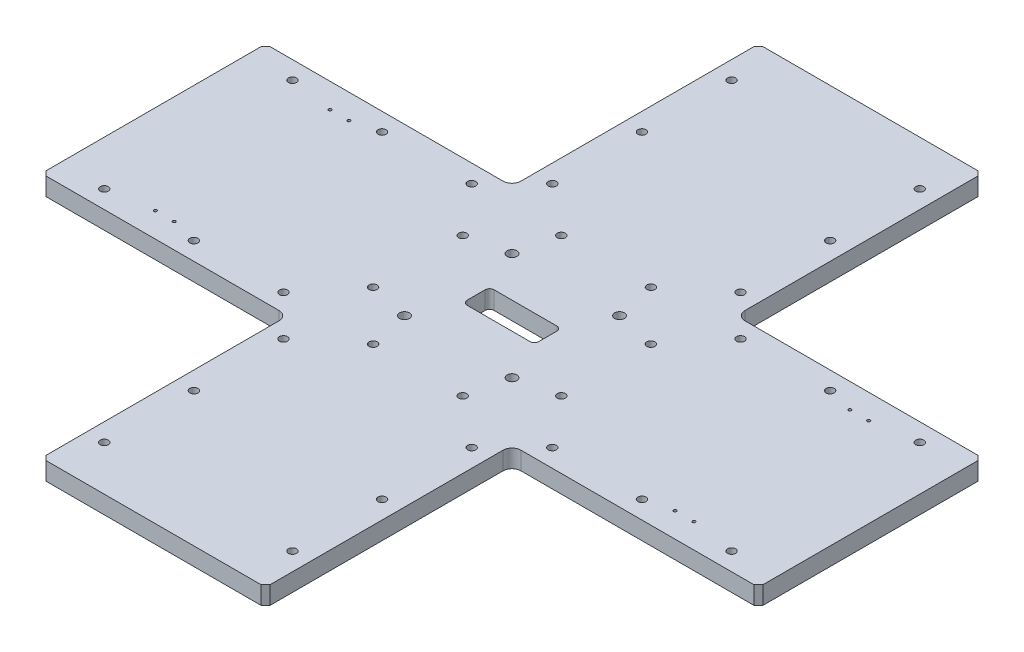
from build123d import *

# Parameters (mm, degrees)
EXTRUDE_1_DEPTH              = 20
FILLET_1_R                   = 10
CHAMFER_1_SIZE               = 5
CUT_EXTRUDE_1_DEPTH          = 567.038867923
HOLE_WIZARD_M10_1_D          = 11
HOLE_WIZARD_M8_1_D           = 9
HOLE_WIZARD_M8_1_CBORE_D     = 15
HOLE_WIZARD_M8_1_CBORE_DEPTH = 9
HOLE_WIZARD_M4_1_D           = 3.3


with BuildPart() as part:
    # 草图1 → 凸台-拉伸1 (new body)
    with BuildSketch(Plane(origin=(0, 0, 0), x_dir=(1, 0, 0), z_dir=(0, 1, 0))):
        Polygon((-125, 125), (-125, 400), (125, 400), (125, 125), (400, 125), (400, -125), (125, -125), (125, -400), (-125, -400), (-125, -125), (-400, -125), (-400, 125), align=None)
    extrude(amount=EXTRUDE_1_DEPTH)

    # 圆角1
    fillet_1_edges = [part.edges().sort_by_distance(p)[0] for p in [
        (-125, 10, 125),
        (-125, 10, -125),
        (125, 10, -125),
        (125, 10, 125),
    ]]
    fillet(fillet_1_edges, radius=FILLET_1_R)

    # 倒角1
    chamfer_1_edges = [part.edges().sort_by_distance(p)[0] for p in [
        (-400, 10, 125),
        (-400, 10, -125),
        (-125, 10, -400),
        (125, 10, -400),
        (400, 10, -125),
        (400, 10, 125),
        (125, 10, 400),
        (-125, 10, 400),
    ]]
    chamfer(chamfer_1_edges, length=CHAMFER_1_SIZE)

    # 草图2 → 切除-拉伸1 (cut, through all)
    with BuildSketch(Plane.XZ):
        with BuildLine():
            Line((-35, 15), (35, 15))
            ThreePointArc((35, 15), (38.535533906, 13.535533906), (40, 10))
            Line((40, 10), (40, -10))
            ThreePointArc((40, -10), (38.535533906, -13.535533906), (35, -15))
            Line((35, -15), (-35, -15))
            ThreePointArc((-35, -15), (-38.535533906, -13.535533906), (-40, -10))
            Line((-40, -10), (-40, 10))
            ThreePointArc((-40, 10), (-38.535533906, 13.535533906), (-35, 15))
        make_face()
    extrude(amount=-CUT_EXTRUDE_1_DEPTH, mode=Mode.SUBTRACT)

    # M10 间隙孔1 (through all)
    with Locations(Plane(origin=(0, 20, 0), x_dir=(1, 0, 0), z_dir=(0, 1, 0))):
        with Locations((-60, 60), (60, 60), (60, -60), (-60, -60)):
            Hole(HOLE_WIZARD_M10_1_D / 2)

    # M8 六角圆柱头螺钉的柱形沉头孔1 (through all)
    with Locations(Plane(origin=(0, 0, 0), x_dir=(-1, 0, 0), z_dir=(0, -1, 0))):
        with Locations((-105, 350), (-105, 250), (-105, 150), (-105, 50), (-350, 105), (-250, 105), (-150, 105), (-50, 105), (50, 105), (150, 105), (250, 105), (350, 105), (105, 50), (105, 150), (105, 250), (105, 350), (0, 0), (105, -350), (105, -250), (105, -150), (105, -50), (350, -105), (250, -105), (150, -105), (50, -105), (-50, -105), (-150, -105), (-250, -105), (-350, -105), (-105, -50), (-105, -150), (-105, -250), (-105, -350)):
            CounterBoreHole(HOLE_WIZARD_M8_1_D / 2, HOLE_WIZARD_M8_1_CBORE_D / 2, HOLE_WIZARD_M8_1_CBORE_DEPTH)

    # M4 螺纹孔1 (through all)
    with Locations(Plane(origin=(0, 0, 0), x_dir=(-1, 0, 0), z_dir=(0, -1, 0))):
        with Locations((-300.5, 97.5), (-279.5, 97.5), (-279.5, -97.5), (-300.5, -97.5), (300.5, -97.5), (279.5, -97.5), (279.5, 97.5), (300.5, 97.5)):
            Hole(HOLE_WIZARD_M4_1_D / 2)


solid = part.part
